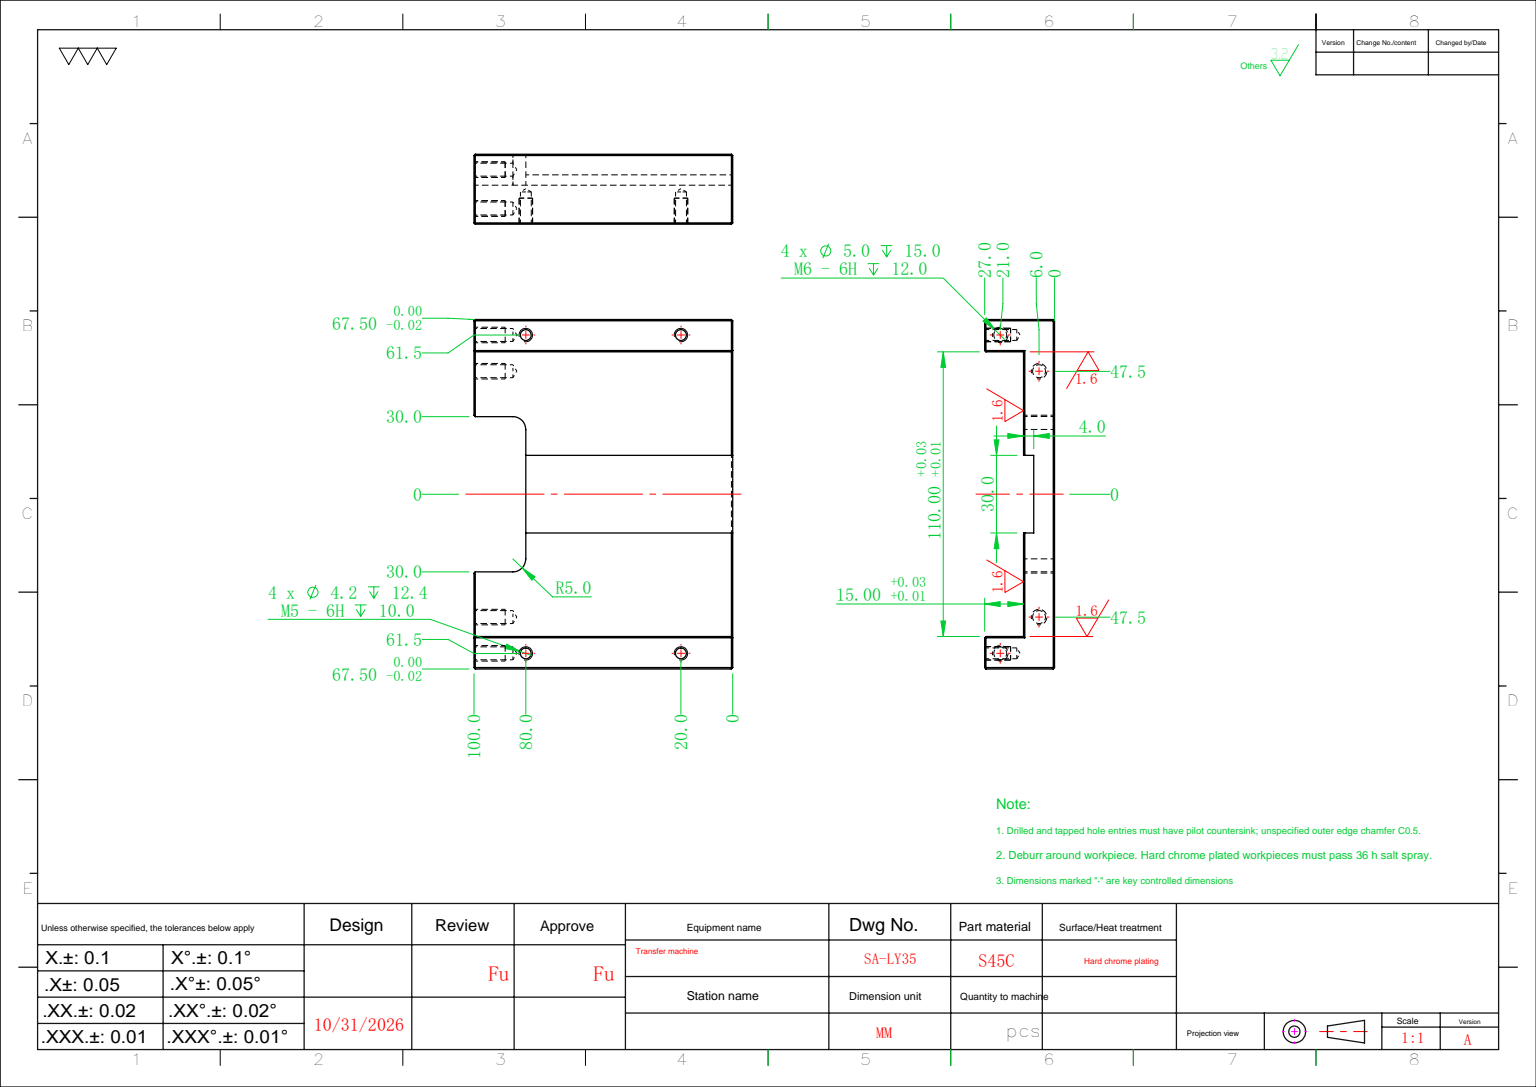
SolidWorks part; units mm, degrees
ref_plane "前视基准面" through (0, 0, 0) normal (0, 0, 1) x (1, 0, 0)
ref_plane "上视基准面" through (0, 0, 0) normal (0, 1, 0) x (1, 0, 0)
ref_plane "右视基准面" through (0, 0, 0) normal (1, 0, 0) x (0, 0, -1)
sketch "草图1" plane through (0, 0, 0) normal (0, 0, 1) x (1, 0, 0)
  line L1 (-67.5, -50) -> (67.5, -50)
  line L2 (-67.5, -50) -> (-67.5, 50)
  line L3 (-67.5, 50) -> (67.5, 50)
  line L4 (67.5, -50) -> (67.5, 50)
  line L5 (-67.5, -50) -> (67.5, 50) construction
  line L6 (-67.5, 50) -> (67.5, -50) construction
  point P0 (0, 0)
  dimension "D1" = 135
  dimension "D2" = 100
extrude "凸台-拉伸1" add sketch "草图1" along normal blind 12
sketch "草图2" plane through (0, 0, 12) normal (0, 0, 1) x (1, 0, 0)
  line L0 (-67.5, -50) -> (67.5, -50) construction
  line L1 (-67.5, 50) -> (-55, 50)
  line L2 (-67.5, 50) -> (-67.5, -50)
  line L3 (-67.5, -50) -> (-55, -50)
  line L4 (-55, 50) -> (-55, -50)
  line L5 (0, 0) -> (0, 57.6018) construction
  line L6 (55, 50) -> (55, -50)
  line L7 (67.5, -50) -> (55, -50)
  line L8 (67.5, 50) -> (67.5, -50)
  line L9 (67.5, 50) -> (55, 50)
  dimension "D1" = 110
extrude "凸台-拉伸2" add sketch "草图2" along normal blind 15
sketch "草图3" plane through (0, 0, 12) normal (0, 0, 1) x (1, 0, 0)
  line L0 (55, 50) -> (-55, 50) construction
  line L1 (-15, -50) -> (15, -50)
  line L2 (-15, -50) -> (-15, 150)
  line L3 (-15, 150) -> (15, 150)
  line L4 (15, -50) -> (15, 150)
  line L5 (-15, -50) -> (15, 150) construction
  line L6 (-15, 150) -> (15, -50) construction
  line L8 (-55, -50) -> (55, -50) construction
  point P0 (0, 50)
  dimension "D1" = 30
extrude "切除-拉伸1" cut sketch "草图3" against normal blind 4
sketch "草图4" plane through (0, 0, 12) normal (0, 0, 1) x (1, 0, 0)
  line L0 (-15, 50) -> (-55, 50) construction
  line L1 (-30, 50) -> (30, 50)
  line L2 (-30, 50) -> (-30, 30)
  line L3 (-30, 30) -> (30, 30)
  line L4 (30, 50) -> (30, 30)
  line L5 (0, 0) -> (0, 64.2894) construction
  dimension "D1" = 60
  dimension "D2" = 20
extrude "切除-拉伸2" cut sketch "草图4" against normal through all
fillet "圆角1" radius 5 2 edges at (-30, 30, 6) (30, 30, 6)
hole_wizard "M6 螺纹孔1" positions "草图5" profile "草图7" tap size "M6" standard "ISO"
sketch "草图5" plane through (0, 50, 0) normal (0, 1, 0) x (1, 0, 0)
  line L0 (0, 0) -> (0, -43.1416) construction
  line L2 (30, -6) -> (-82.4308, -6) construction
  line L3 (30, 0) -> (30, -12) construction
  point P0 (-61.5, -21)
  point P2 (-47.5, -6)
  point P11 (47.5, -6)
  point P12 (61.5, -21)
  dimension "D1" = 95
  dimension "D2" = 123
  dimension "D3" = 15
sketch "草图7" plane through (-61.5, 50, 21) normal (1, 0, 0) x (0, 0, 1)
  line L0 (0, 0) -> (0, 16.5022)
  line L1 (0, 16.5022) -> (2.5, 15)
  line L2 (2.5, 15) -> (2.5, 0)
  line L5 (2.5, 0) -> (0, 0)
  line L10 (0, 16.5022) -> (-2.5, 15) construction
  line L11 (0, -6.35) -> (0, 107.95) construction
  dimension "螺纹孔钻头直径" = 5
  dimension "螺纹孔钻头深度" = 15
  dimension "导头角度" = 118
cosmetic thread "孔螺蚊线2" parameters "D1"=12, "D2"=6
cosmetic thread "孔螺蚊线3" parameters "D1"=12, "D2"=6
cosmetic thread "孔螺蚊线8" parameters "D1"=12, "D2"=6
cosmetic thread "孔螺蚊线9" parameters "D1"=12, "D2"=6
hole_wizard "M5 螺纹孔1" positions "草图8" profile "草图9" tap size "M5" standard "ISO"
sketch "草图8" plane through (0, 0, 27) normal (0, 0, 1) x (1, 0, 0)
  line L0 (0, 0) -> (0, -62.2913) construction
  line L2 (-67.5, -50) -> (67.5, -50) construction
  point P0 (-61.5, 30)
  point P3 (-61.5, -30)
  point P16 (61.5, -30)
  point P17 (61.5, 30)
  dimension "D1" = 123
  dimension "D2" = 20
  dimension "D3" = 60
sketch "草图9" plane through (-61.5, 30, 27) normal (1, 0, 0) x (0, -1, 0)
  line L0 (0, 0) -> (0, 13.6618)
  line L1 (0, 13.6618) -> (2.1, 12.4)
  line L2 (2.1, 12.4) -> (2.1, 0)
  line L5 (2.1, 0) -> (0, 0)
  line L10 (0, 13.6618) -> (-2.1, 12.4) construction
  line L11 (0, -6.35) -> (0, 107.95) construction
  dimension "螺纹孔钻头直径" = 4.2
  dimension "螺纹孔钻头深度" = 12.4
  dimension "导头角度" = 118
cosmetic thread "孔螺蚊线4" parameters "D1"=10, "D2"=5.2
cosmetic thread "孔螺蚊线5" parameters "D1"=10, "D2"=5.2
cosmetic thread "孔螺蚊线6" parameters "D1"=10, "D2"=5.2
cosmetic thread "孔螺蚊线7" parameters "D1"=10, "D2"=5.2
chamfer "倒角1" distance 0.5 angle 45 27 edges at (-35, -50, 12) (-55, -50, 19.5) (-55, 50, 19.5) (-67.5, 0, 27) (-61.25, -50, 27) (-55, 0, 27) (-61.25, 50, 27) (42.5, 50, 12) (55, 50, 19.5) (55, -50, 19.5) (61.25, 50, 27) (55, 0, 27) (61.25, -50, 27) (67.5, 0, 27) (35, -50, 12) (0, -50, 0) (-67.5, 0, 0) (48.75, 50, 0) (67.5, 0, 0) (-48.75, 50, 0) (-42.5, 50, 12) (-30, 50, 6) (30, 50, 6) (67.5, -50, 13.5) (-67.5, -50, 13.5) (-67.5, 50, 13.5) (67.5, 50, 13.5)
